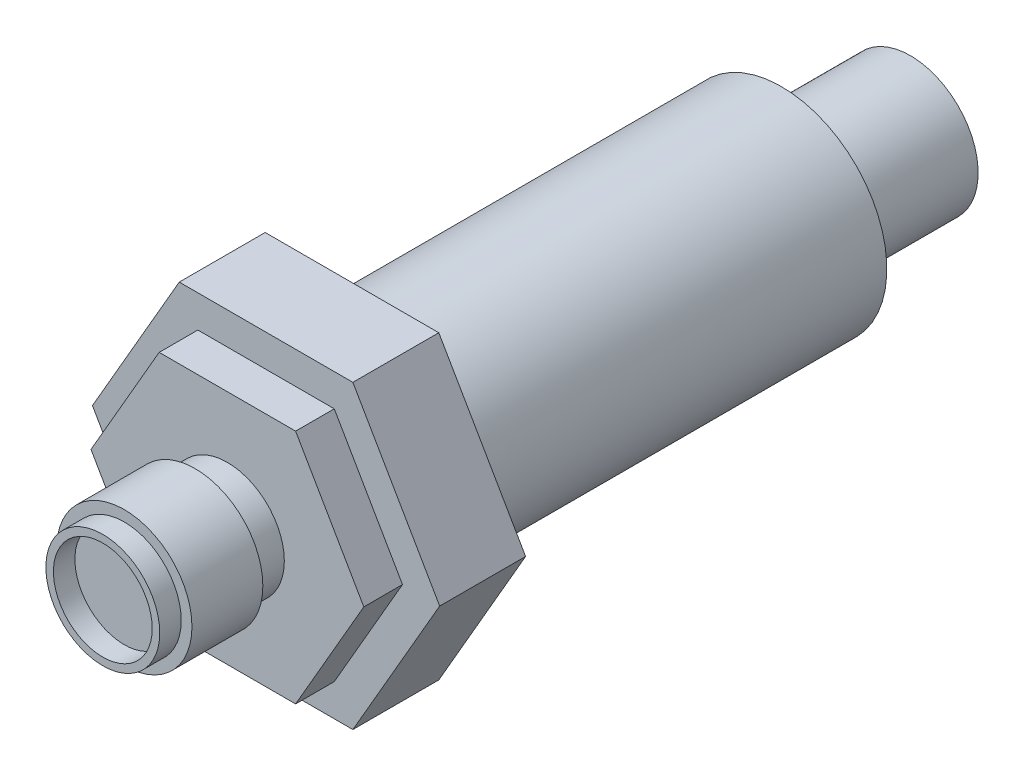
from build123d import *

# Parameters (mm, degrees)
BOSS_EXTRUDE1_DEPTH = 4
BOSS_EXTRUDE2_DEPTH = 1.8
SKETCH3_R           = 2.65
SKETCH3_R_2         = 2.3
BOSS_EXTRUDE3_DEPTH = 5.8
BOSS_EXTRUDE4_START = -1
SKETCH4_R           = 3.15
BOSS_EXTRUDE4_DEPTH = 3.3
SKETCH5_R           = 4.9
BOSS_EXTRUDE5_DEPTH = 20
SKETCH6_R           = 3.15
SKETCH6_R_2         = 2.25
BOSS_EXTRUDE6_DEPTH = 6


with BuildPart() as part:
    # Sketch1 → Boss-Extrude1 (new body)
    with BuildSketch(Plane.XY):
        Polygon((8.082903769, 0), (4.041451884, 7), (-4.041451884, 7), (-8.082903769, 0), (-4.041451884, -7), (4.041451884, -7), align=None)
    extrude(amount=BOSS_EXTRUDE1_DEPTH)

    # Sketch2 → Boss-Extrude2 (add)
    with BuildSketch(Plane.XY.offset(4)):
        Polygon((6.350852961, 0), (3.175426481, 5.5), (-3.175426481, 5.5), (-6.350852961, 0), (-3.175426481, -5.5), (3.175426481, -5.5), align=None)
    extrude(amount=BOSS_EXTRUDE2_DEPTH)

    # Sketch3 → Boss-Extrude3 (add)
    with BuildSketch(Plane.XY.offset(5.8)):
        Circle(SKETCH3_R)
        Circle(SKETCH3_R_2, mode=Mode.SUBTRACT)
    extrude(amount=BOSS_EXTRUDE3_DEPTH)

    # Sketch4 → Boss-Extrude4 (add)
    with BuildSketch(Plane.XY.offset(11.6).offset(BOSS_EXTRUDE4_START)):
        Circle(SKETCH4_R)
    extrude(amount=-BOSS_EXTRUDE4_DEPTH)

    # Sketch5 → Boss-Extrude5 (add)
    with BuildSketch(Plane(origin=(0, 0, 0), x_dir=(-1, 0, 0), z_dir=(0, 0, -1))):
        Circle(SKETCH5_R)
    extrude(amount=BOSS_EXTRUDE5_DEPTH)

    # Sketch6 → Boss-Extrude6 (add)
    with BuildSketch(Plane(origin=(0, 0, -20), x_dir=(-1, 0, 0), z_dir=(0, 0, -1))):
        with Locations(Location((0, 0, 0), (0, 0, 180))):
            Circle(SKETCH6_R)
        Circle(SKETCH6_R_2, mode=Mode.SUBTRACT)
    extrude(amount=BOSS_EXTRUDE6_DEPTH)


solid = part.part
